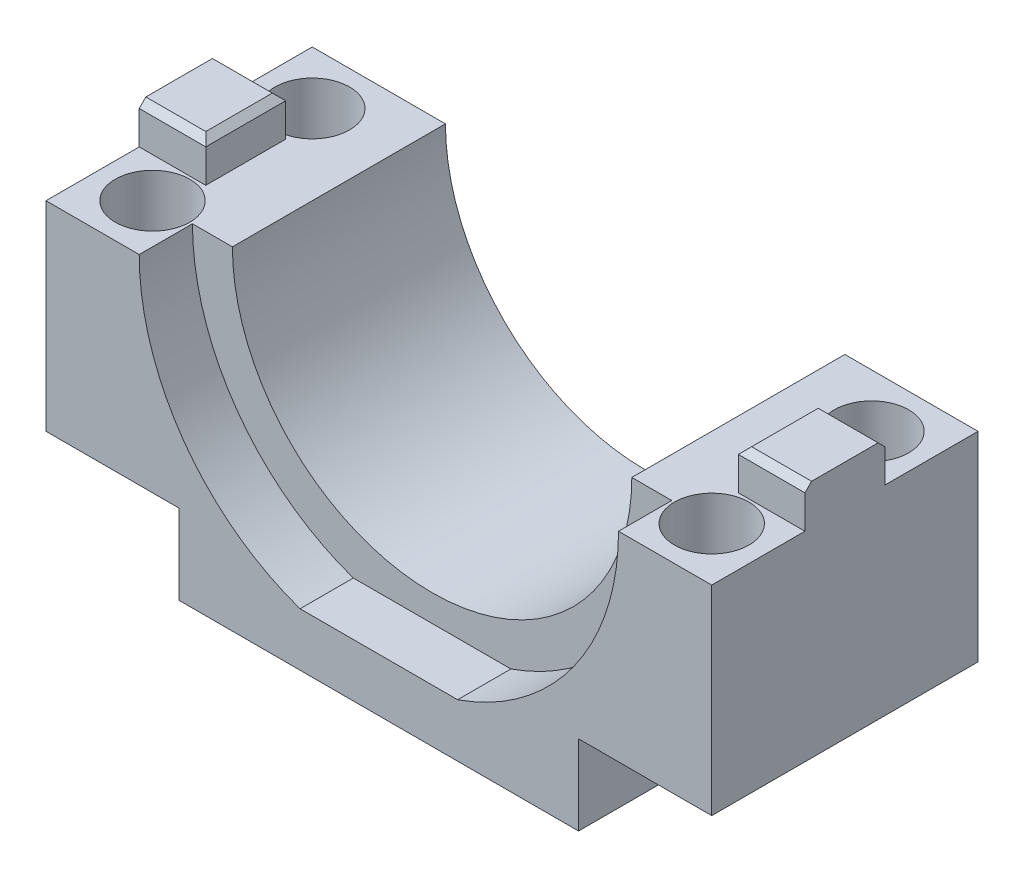
from build123d import *

# Parameters (mm, degrees)
SKETCH1_W           = 50
SKETCH1_H           = 21
BOSS_EXTRUDE1_DEPTH = 20
SKETCH2_R           = 15
CUT_EXTRUDE1_DEPTH  = 20
SKETCH3_W           = 10
SKETCH3_H           = 6
CUT_EXTRUDE2_DEPTH  = 20
SKETCH4_R           = 2.8
CUT_EXTRUDE3_DEPTH  = 20
SKETCH5_W           = 5
SKETCH5_H           = 6
BOSS_EXTRUDE2_DEPTH = 3
CHAMFER2_SIZE       = 0.5
CUT_EXTRUDE4_DEPTH  = 4


with BuildPart() as part:
    # Sketch1 → Boss-Extrude1 (new body)
    with BuildSketch(Plane.XY):
        Rectangle(SKETCH1_W, SKETCH1_H)
    extrude(amount=BOSS_EXTRUDE1_DEPTH)

    # Sketch2 → Cut-Extrude1 (cut)
    with BuildSketch(Plane.XY.offset(20)):
        with Locations((0, 10.5)):
            Circle(SKETCH2_R)
    extrude(amount=-CUT_EXTRUDE1_DEPTH, mode=Mode.SUBTRACT)

    # Sketch3 → Cut-Extrude2 (cut)
    with BuildSketch(Plane.XY.offset(20)):
        with Locations((-20, -7.5)):
            Rectangle(SKETCH3_W, SKETCH3_H)
        with Locations((20, -7.5)):
            Rectangle(SKETCH3_W, SKETCH3_H)
    extrude(amount=-CUT_EXTRUDE2_DEPTH, mode=Mode.SUBTRACT)

    # Sketch4 → Cut-Extrude3 (cut)
    with BuildSketch(Plane.XZ.offset(4.5)):
        with Locations((-21, 16)):
            Circle(SKETCH4_R)
        with Locations((-21, 4)):
            Circle(SKETCH4_R)
        with Locations((21, 16)):
            Circle(SKETCH4_R)
        with Locations((21, 4)):
            Circle(SKETCH4_R)
    extrude(amount=-CUT_EXTRUDE3_DEPTH, mode=Mode.SUBTRACT)

    # Sketch5 → Boss-Extrude2 (add)
    with BuildSketch(Plane(origin=(0, 10.5, 0), x_dir=(1, 0, 0), z_dir=(0, 1, 0))):
        with Locations((-22.5, -10)):
            Rectangle(SKETCH5_W, SKETCH5_H)
        with Locations((22.5, -10)):
            Rectangle(SKETCH5_W, SKETCH5_H)
    extrude(amount=BOSS_EXTRUDE2_DEPTH)

    # Chamfer2
    chamfer2_edges = [part.edges().sort_by_distance(p)[0] for p in [
        (-22.5, 13.5, 13),
        (-20, 13.5, 10),
        (-22.5, 13.5, 7),
        (20, 13.5, 10),
        (22.5, 13.5, 13),
        (22.5, 13.5, 7),
    ]]
    chamfer(chamfer2_edges, length=CHAMFER2_SIZE)

    # Sketch6 → Cut-Extrude4 (cut)
    with BuildSketch(Plane.XY.offset(20)):
        with BuildLine():
            Line((-5.916079783, -6.5), (5.916079783, -6.5))
            ThreePointArc((5.916079783, -6.5), (0, 28.5), (-5.916079783, -6.5))
        make_face()
    extrude(amount=-CUT_EXTRUDE4_DEPTH, mode=Mode.SUBTRACT)


solid = part.part
